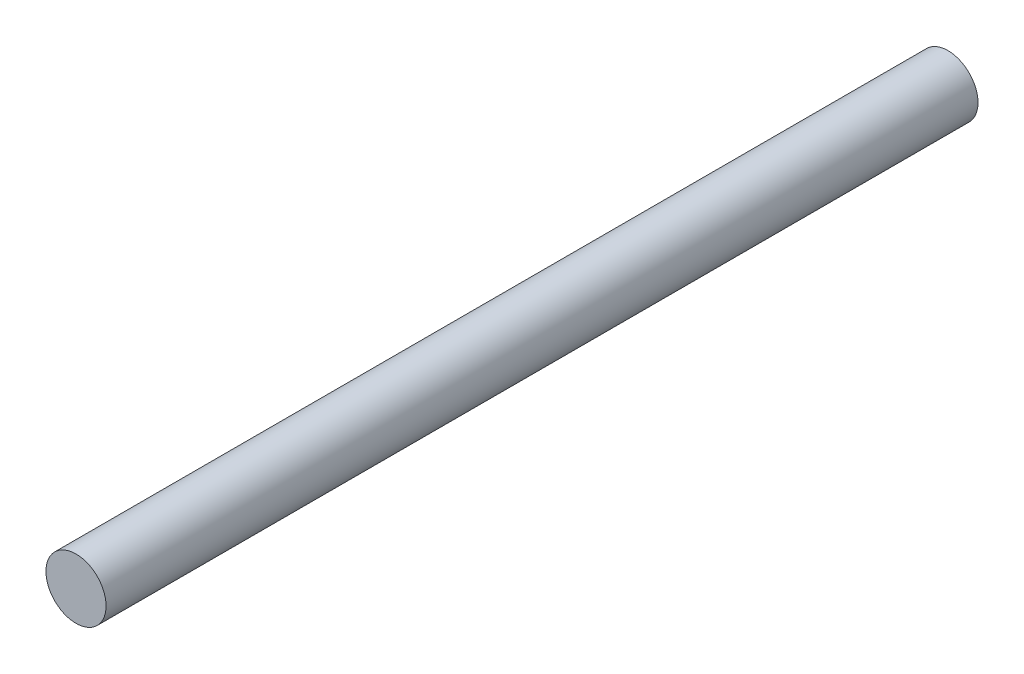
SolidWorks part; units mm, degrees
ref_plane "前视基准面" through (0, 0, 0) normal (0, 0, 1) x (1, 0, 0)
ref_plane "上视基准面" through (0, 0, 0) normal (0, 1, 0) x (1, 0, 0)
ref_plane "右视基准面" through (0, 0, 0) normal (1, 0, 0) x (0, 0, -1)
sketch "草图1" plane through (0, 0, 0) normal (0, 0, 1) x (1, 0, 0)
  circle A0 centre (0, 0) radius 10
  dimension "D1" = 20
extrude "凸台-拉伸1" add sketch "草图1" along normal mid plane 290
